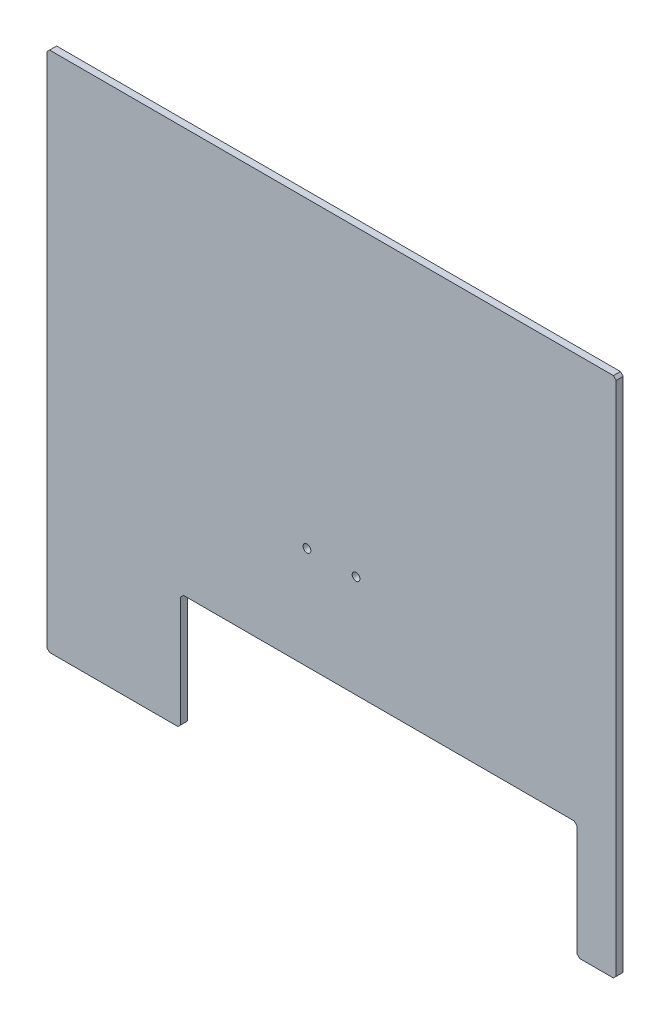
SolidWorks part; units mm, degrees
material "PC "
ref_plane "Front Plane" through (0, 0, 0) normal (0, 0, 1) x (1, 0, 0)
ref_plane "Top Plane" through (0, 0, 0) normal (0, 1, 0) x (1, 0, 0)
ref_plane "Right Plane" through (0, 0, 0) normal (1, 0, 0) x (0, 0, -1)
sketch "Sketch1" plane through (0, 0, 0) normal (0, 0, 1) x (1, 0, 0)
  line L1 (203, -186) -> (-203, -186)
  line L2 (203, -186) -> (203, 186)
  line L3 (203, 186) -> (-203, 186)
  line L4 (-203, -186) -> (-203, 186)
  line L5 (203, -186) -> (-203, 186) construction
  line L6 (203, 186) -> (-203, -186) construction
  point P0 (0, 0)
  dimension "D1" = 406
  dimension "D2" = 372
extrude "Boss-Extrude1" add sketch "Sketch1" along normal blind 5
sketch "Sketch2" plane through (0, 0, 5) normal (0, 0, 1) x (1, 0, 0)
  line L0 (0, 0) -> (0, -148.0944) construction
  line L2 (175, -186) -> (-107.5, -186)
  line L3 (175, -186) -> (175, -103)
  line L4 (175, -103) -> (-107.5, -103)
  line L5 (-107.5, -186) -> (-107.5, -103)
  line L8 (-203, -186) -> (203, -186) construction
  point P3 (0, -136)
  dimension "D1" = 107.5
  dimension "D2" = 83
  dimension "D3" = 175
extrude "Cut-Extrude1" cut sketch "Sketch2" against normal through all
hole_wizard "M5 Clearance Hole1" positions "Sketch5" profile "Sketch4" hole size "M5" standard "GB" end condition up to next
sketch "Sketch5" plane through (0, 0, 5) normal (0, 0, 1) x (1, 0, 0)
  line L0 (0, 161.3177) -> (0, 0) construction
  line L1 (0, 0) -> (-168.4712, 0) construction
  line L4 (203, 186) -> (-203, 186) construction
  point P0 (-17.5, -30)
  point P12 (17.5, -30)
  dimension "D1" = 17.5
  dimension "D2" = 216
sketch "Sketch4" plane through (-17.5, -30, 5) normal (1, 0, 0) x (0, -1, 0)
  line L0 (0, 0) -> (0, 5)
  line L1 (0, 5) -> (2.75, 5)
  line L2 (2.75, 5) -> (2.75, 0)
  line L5 (2.75, 0) -> (0, 0)
  line L11 (0, -6.35) -> (0, 107.95) construction
  dimension "通孔孔直径" = 5.5
  dimension "通孔孔深度" = 5
fillet "Fillet1" radius 2 8 edges at (-203, 186, 2.5) (203, 186, 2.5) (203, -186, 2.5) (-203, -186, 2.5) (175, -103, 2.5) (-107.5, -103, 2.5) (175, -186, 2.5) (-107.5, -186, 2.5) profile chamfer
